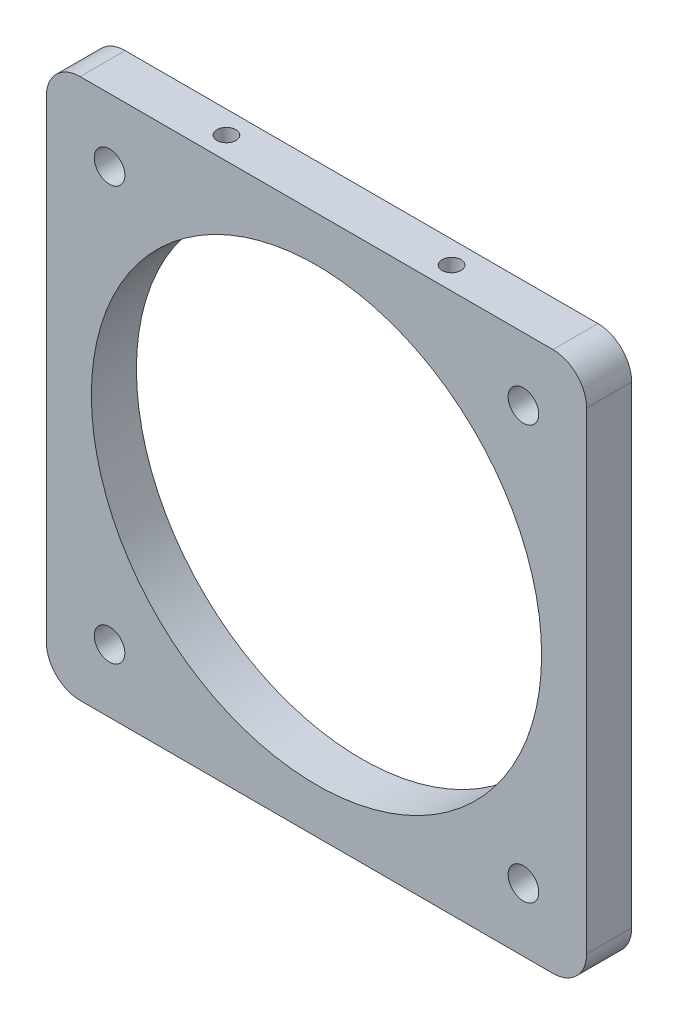
SolidWorks part; units mm, degrees
ref_plane "Front Plane" through (0, 0, 0) normal (0, 0, 1) x (1, 0, 0)
ref_plane "Top Plane" through (0, 0, 0) normal (0, 1, 0) x (1, 0, 0)
ref_plane "Right Plane" through (0, 0, 0) normal (1, 0, 0) x (0, 0, -1)
sketch "Sketch1" plane through (0, 0, 0) normal (0, 0, 1) x (1, 0, 0)
  line L1 (60, -60) -> (-60, -60)
  line L2 (60, -60) -> (60, 60)
  line L3 (60, 60) -> (-60, 60)
  line L4 (-60, -60) -> (-60, 60)
  line L5 (60, -60) -> (-60, 60) construction
  line L6 (60, 60) -> (-60, -60) construction
  point P0 (0, 0)
  dimension "D1" = 120
  dimension "D2" = 120
extrude "Boss-Extrude1" add sketch "Sketch1" along normal blind 10
fillet "Fillet1" radius 7.5 4 edges at (-60, -60, 5) (60, -60, 5) (60, 60, 5) (-60, 60, 5)
hole_wizard "M5 Tapped Hole1" positions "Sketch2" profile "Sketch3" tap size "M5" standard "GB"
sketch "Sketch2" plane through (0, 60, 0) normal (0, 1, 0) x (1, 0, 0)
  line L0 (52.5, 0) -> (-52.5, 0) construction
  point P0 (-25, -5)
  point P2 (25, -5)
  dimension "D1" = 5
  dimension "D2" = 50
  dimension "D3" = 25
sketch "Sketch3" plane through (-25, 60, 5) normal (1, 0, 0) x (0, 0, 1)
  line L0 (0, 0) -> (0, 13.6618)
  line L1 (0, 13.6618) -> (2.1, 12.4)
  line L2 (2.1, 12.4) -> (2.1, 0)
  line L5 (2.1, 0) -> (0, 0)
  line L10 (0, 13.6618) -> (-2.1, 12.4) construction
  line L11 (0, -6.35) -> (0, 107.95) construction
  dimension "螺纹孔钻头直径" = 4.2
  dimension "螺纹孔钻头深度" = 12.4
  dimension "导头角度" = 118
cosmetic thread "Cosmetic Thread1" parameters "D1"=10, "D2"=5
cosmetic thread "Cosmetic Thread2" parameters "D1"=10, "D2"=5
sketch "Sketch4" plane through (0, 0, 10) normal (0, 0, 1) x (1, 0, 0)
  circle A0 centre (0, 0) radius 50
  dimension "D1" = 100
extrude "Cut-Extrude1" cut sketch "Sketch4" against normal blind 10
sketch "Sketch5" plane through (0, 0, 10) normal (0, 0, 1) x (1, 0, 0)
  line L1 (45.9619, -45.9619) -> (-45.9619, -45.9619)
  line L2 (45.9619, -45.9619) -> (45.9619, 45.9619)
  line L3 (45.9619, 45.9619) -> (-45.9619, 45.9619)
  line L4 (-45.9619, -45.9619) -> (-45.9619, 45.9619)
  line L5 (45.9619, -45.9619) -> (-45.9619, 45.9619) construction
  line L6 (45.9619, 45.9619) -> (-45.9619, -45.9619) construction
  circle A0 centre (0, 0) radius 65
  point P0 (0, 0)
  dimension "D1" = 130
hole_wizard "M8 Tapped Hole1" positions "Sketch6" profile "Sketch7" tap size "M8" standard "GB"
sketch "Sketch6" plane through (0, 0, 10) normal (0, 0, 1) x (1, 0, 0)
  point P0 (-45.9619, 45.9619)
  point P3 (45.9619, 45.9619)
  point P6 (45.9619, -45.9619)
  point P9 (-45.9619, -45.9619)
sketch "Sketch7" plane through (-45.9619, 45.9619, 10) normal (1, 0, 0) x (0, -1, 0)
  line L0 (0, 0) -> (0, 21.7929)
  line L1 (0, 21.7929) -> (3.4, 19.75)
  line L2 (3.4, 19.75) -> (3.4, 0)
  line L5 (3.4, 0) -> (0, 0)
  line L10 (0, 21.7929) -> (-3.4, 19.75) construction
  line L11 (0, -6.35) -> (0, 107.95) construction
  dimension "螺纹孔钻头直径" = 6.8
  dimension "螺纹孔钻头深度" = 19.75
  dimension "导头角度" = 118
cosmetic thread "Cosmetic Thread3" parameters "D1"=10, "D2"=8
cosmetic thread "Cosmetic Thread4" parameters "D1"=10, "D2"=8
cosmetic thread "Cosmetic Thread5" parameters "D1"=10, "D2"=8
cosmetic thread "Cosmetic Thread6" parameters "D1"=10, "D2"=8
